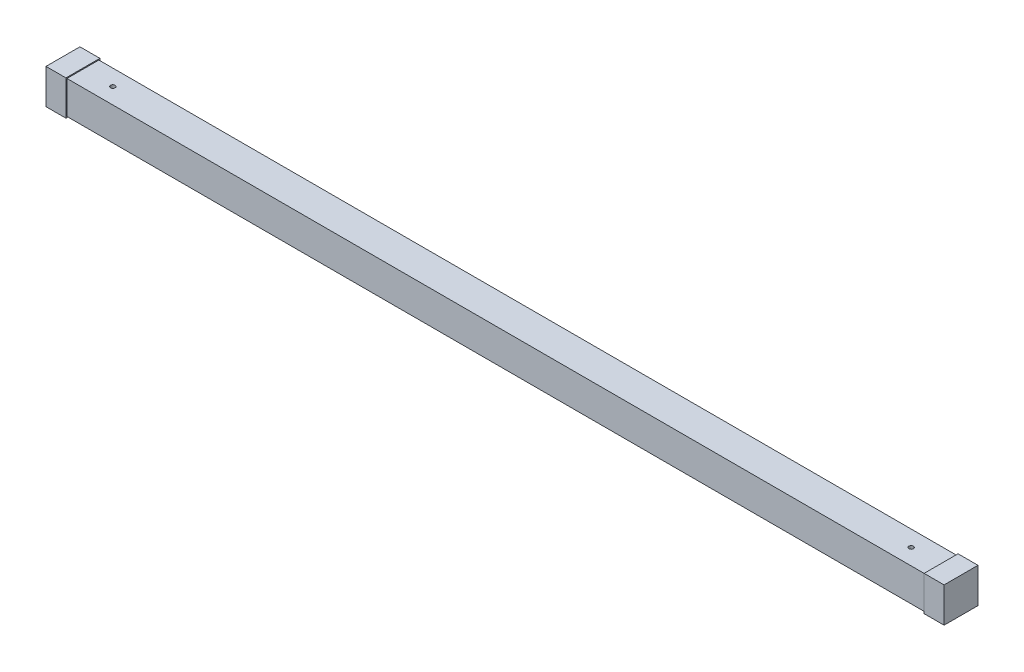
SolidWorks part; units mm, degrees
ref_plane "前视基准面" through (0, 0, 0) normal (0, 0, 1) x (1, 0, 0)
ref_plane "上视基准面" through (0, 0, 0) normal (0, 1, 0) x (1, 0, 0)
ref_plane "右视基准面" through (0, 0, 0) normal (1, 0, 0) x (0, 0, -1)
sketch "草图1" plane through (0, 0, 0) normal (0, 0, 1) x (1, 0, 0)
  line L1 (-450, 16.5) -> (450, 16.5)
  line L2 (-450, 16.5) -> (-450, -16.5)
  line L3 (-450, -16.5) -> (450, -16.5)
  line L4 (450, 16.5) -> (450, -16.5)
  line L5 (-450, 16.5) -> (450, -16.5) construction
  line L6 (-450, -16.5) -> (450, 16.5) construction
  point P0 (0, 0)
  dimension "D1" = 900
  dimension "D2" = 33
extrude "凸台-拉伸1" add sketch "草图1" along normal mid plane 32
sketch "草图2" plane through (450, 0, 0) normal (1, 0, 0) x (0, 0, -1)
  line L0 (-16, 16.5) -> (16, 16.5) construction
  line L1 (-17, 17.5) -> (17, 17.5)
  line L2 (-17, 17.5) -> (-17, -17.5)
  line L3 (-17, -17.5) -> (17, -17.5)
  line L4 (17, 17.5) -> (17, -17.5)
  line L5 (-17, 17.5) -> (17, -17.5) construction
  line L6 (-17, -17.5) -> (17, 17.5) construction
  line L7 (-16, -16.5) -> (-16, 16.5) construction
  point P0 (0, 0)
  dimension "D1" = 1
  dimension "D2" = 1
extrude "凸台-拉伸2" add sketch "草图2" against normal blind 20
mirror "镜向2" about plane through (0, 0, 0) normal (1, 0, 0) of "凸台-拉伸2"
hole_wizard "Ø4.5 (4.5) 直径孔1" positions "草图3" profile "草图4" hole size "Ø4.5" standard "GB"
sketch "草图3" plane through (0, 16.5, 0) normal (0, 1, 0) x (1, 0, 0)
  line L0 (-400, 0) -> (400, 0) construction
  point P0 (-400, 0)
  point P2 (400, 0)
  dimension "D1" = 800
sketch "草图4" plane through (-400, 16.5, 0) normal (1, 0, 0) x (0, 0, 1)
  line L0 (0, 0) -> (0, 11.3519)
  line L1 (0, 11.3519) -> (2.25, 10)
  line L2 (2.25, 10) -> (2.25, 0)
  line L5 (2.25, 0) -> (0, 0)
  line L10 (0, 11.3519) -> (-2.25, 10) construction
  line L11 (0, -6.35) -> (0, 107.95) construction
  dimension "孔直径" = 4.5
  dimension "孔深度" = 10
  dimension "导头角度" = 118
